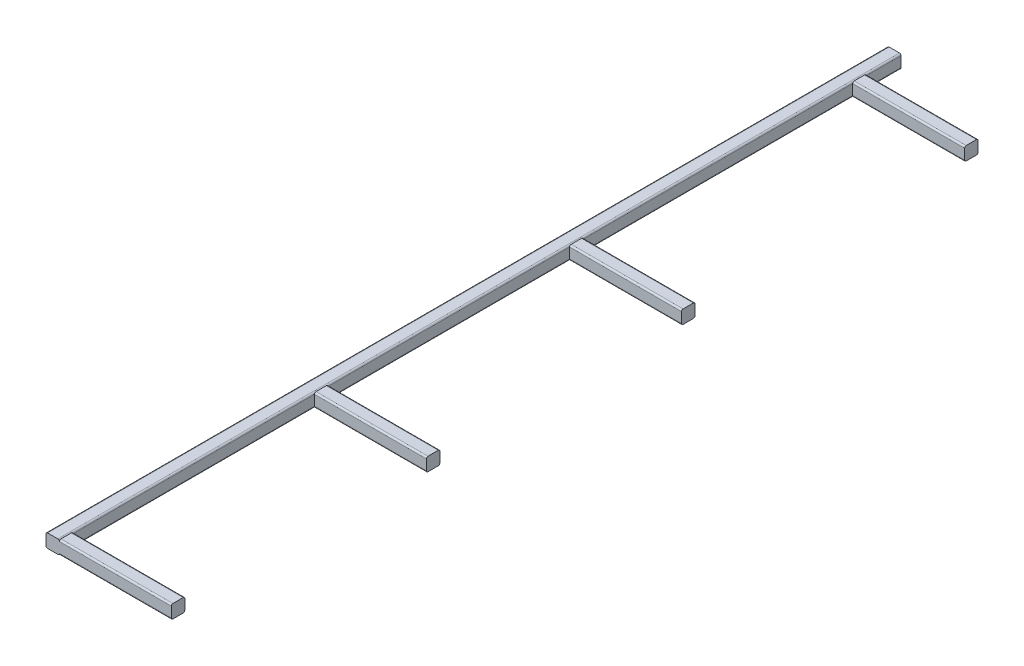
from build123d import *

# Parameters (mm, degrees)
BOSS_EXTRUDE1_DEPTH = 1880
BOSS_EXTRUDE2_DEPTH = 250


with BuildPart() as part:
    # Sketch1 → Boss-Extrude1 (new body)
    with BuildSketch(Plane.XY):
        with BuildLine():
            Line((3.5, 0), (26.5, 0))
            ThreePointArc((26.5, 0), (28.974873734, -1.025126266), (30, -3.5))
            Line((30, -3.5), (30, -26.5))
            ThreePointArc((30, -26.5), (28.974873734, -28.974873734), (26.5, -30))
            Line((26.5, -30), (3.5, -30))
            ThreePointArc((3.5, -30), (1.025126266, -28.974873734), (0, -26.5))
            Line((0, -26.5), (0, -3.5))
            ThreePointArc((0, -3.5), (1.025126266, -1.025126266), (3.5, 0))
        make_face()
    extrude(amount=BOSS_EXTRUDE1_DEPTH)

    # Sketch2 → Boss-Extrude2 (add)
    with BuildSketch(Plane(origin=(30, 0, 0), x_dir=(0, 0, -1), z_dir=(1, 0, 0))):
        with BuildLine():
            Line((-1876.5, 0), (-1853.5, 0))
            ThreePointArc((-1853.5, 0), (-1851.025126266, -1.025126266), (-1850, -3.5))
            Line((-1850, -3.5), (-1850, -26.5))
            ThreePointArc((-1850, -26.5), (-1851.025126266, -28.974873734), (-1853.5, -30))
            Line((-1853.5, -30), (-1876.5, -30))
            ThreePointArc((-1876.5, -30), (-1878.974873734, -28.974873734), (-1880, -26.5))
            Line((-1880, -26.5), (-1880, -3.5))
            ThreePointArc((-1880, -3.5), (-1878.974873734, -1.025126266), (-1876.5, 0))
        make_face()
        with BuildLine():
            Line((-104.561536833, 0), (-81.561536833, 0))
            ThreePointArc((-81.561536833, 0), (-79.086663099, -1.025126266), (-78.061536833, -3.5))
            Line((-78.061536833, -3.5), (-78.061536833, -26.5))
            ThreePointArc((-78.061536833, -26.5), (-79.086663099, -28.974873734), (-81.561536833, -30))
            Line((-81.561536833, -30), (-104.561536833, -30))
            ThreePointArc((-104.561536833, -30), (-107.036410567, -28.974873734), (-108.061536833, -26.5))
            Line((-108.061536833, -26.5), (-108.061536833, -3.5))
            ThreePointArc((-108.061536833, -3.5), (-107.036410567, -1.025126266), (-104.561536833, 0))
        make_face()
        with BuildLine():
            Line((-1306.742108749, 0), (-1283.742108749, 0))
            ThreePointArc((-1283.742108749, 0), (-1281.267235014, -1.025126266), (-1280.242108749, -3.5))
            Line((-1280.242108749, -3.5), (-1280.242108749, -26.5))
            ThreePointArc((-1280.242108749, -26.5), (-1281.267235014, -28.974873734), (-1283.742108749, -30))
            Line((-1283.742108749, -30), (-1306.742108749, -30))
            ThreePointArc((-1306.742108749, -30), (-1309.216982483, -28.974873734), (-1310.242108749, -26.5))
            Line((-1310.242108749, -26.5), (-1310.242108749, -3.5))
            ThreePointArc((-1310.242108749, -3.5), (-1309.216982483, -1.025126266), (-1306.742108749, 0))
        make_face()
        with BuildLine():
            Line((-736.86903894, 0), (-713.86903894, 0))
            ThreePointArc((-713.86903894, 0), (-711.394165206, -1.025126266), (-710.36903894, -3.5))
            Line((-710.36903894, -3.5), (-710.36903894, -26.5))
            ThreePointArc((-710.36903894, -26.5), (-711.394165206, -28.974873734), (-713.86903894, -30))
            Line((-713.86903894, -30), (-736.86903894, -30))
            ThreePointArc((-736.86903894, -30), (-739.343912674, -28.974873734), (-740.36903894, -26.5))
            Line((-740.36903894, -26.5), (-740.36903894, -3.5))
            ThreePointArc((-740.36903894, -3.5), (-739.343912674, -1.025126266), (-736.86903894, 0))
        make_face()
    extrude(amount=BOSS_EXTRUDE2_DEPTH)


solid = part.part
